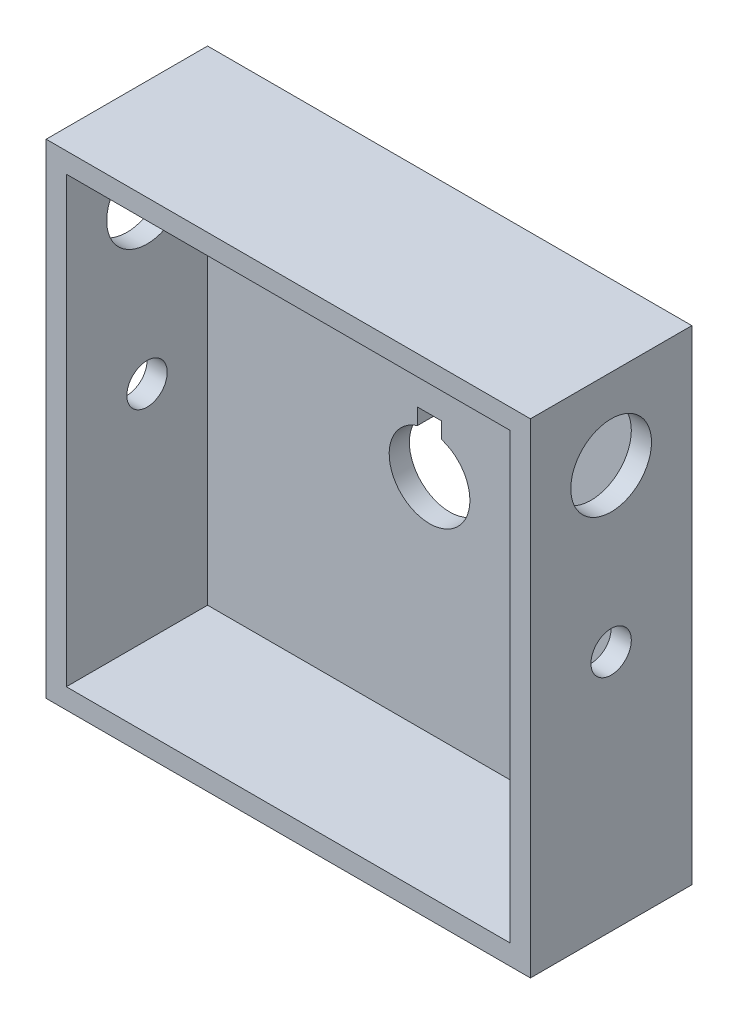
SolidWorks part; units mm, degrees
material "Zoltek Panex 33"
ref_plane "前视基准面" through (0, 0, 0) normal (0, 0, 1) x (1, 0, 0)
ref_plane "上视基准面" through (0, 0, 0) normal (0, 1, 0) x (1, 0, 0)
ref_plane "右视基准面" through (0, 0, 0) normal (1, 0, 0) x (0, 0, -1)
other "Configuration Table"
sketch "草图1" plane through (0, 0, 0) normal (0, 0, 1) x (1, 0, 0)
  line L1 (-60, -60) -> (60, -60)
  line L2 (-60, -60) -> (-60, 60)
  line L3 (-60, 60) -> (60, 60)
  line L4 (60, -60) -> (60, 60)
  line L5 (-60, -60) -> (60, 60) construction
  line L6 (-60, 60) -> (60, -60) construction
  point P0 (0, 0)
  dimension "D1" = 120
  dimension "D2" = 120
extrude "凸台-拉伸1" add sketch "草图1" along normal blind 40
sketch "草图3" plane through (60, 0, 0) normal (1, 0, 0) x (0, 0, -1)
  circle A0 centre (-20, 40) radius 10
  circle A1 centre (-20, 0) radius 5
  dimension "D2" = 20
  dimension "D4" = 10
  dimension "D3" = 40
extrude "切除-拉伸1" cut sketch "草图3" against normal through all
sketch "草图4" plane through (0, 0, 40) normal (0, 0, 1) x (1, 0, 0)
  line L1 (-55, -55) -> (55, -55)
  line L2 (-55, -55) -> (-55, 55)
  line L3 (-55, 55) -> (55, 55)
  line L4 (55, -55) -> (55, 55)
  line L5 (-55, -55) -> (55, 55) construction
  line L6 (-55, 55) -> (55, -55) construction
  point P0 (0, 0)
  dimension "D1" = 110
  dimension "D2" = 110
extrude "切除-拉伸3" cut sketch "草图4" against normal blind 35
sketch "草图5" plane through (0, 0, 0) normal (0, 0, -1) x (-1, 0, 0)
  line L0 (-3, 9.5394) -> (-3, 13.5394)
  line L1 (3, 9.5394) -> (3, 13.5394)
  line L4 (3, 13.5394) -> (-3, 13.5394)
  arc A0 (-3, 9.5394) -> (3, 9.5394) centre (0, 0) ccw
  dimension "D1" = 20
  dimension "D4" = 4
extrude "切除-拉伸4" cut sketch "草图5" against normal through all
